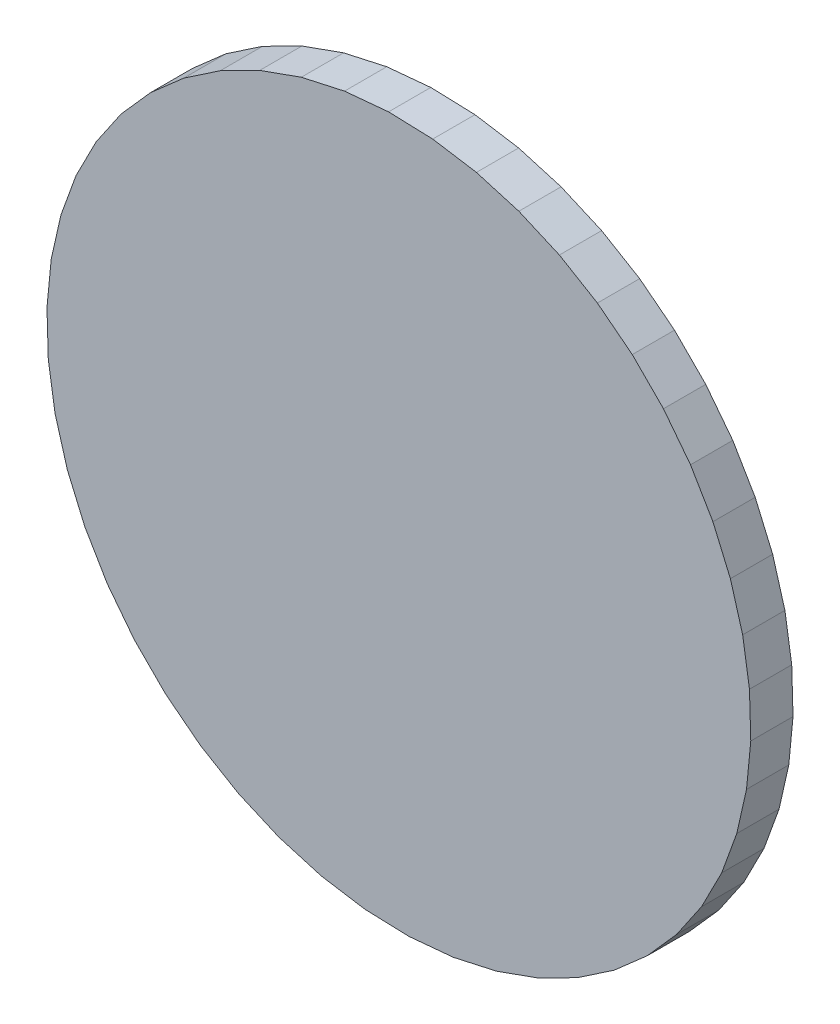
SolidWorks part; units mm, degrees
ref_plane "Front Plane" through (0, 0, 0) normal (0, 0, 1) x (1, 0, 0)
ref_plane "Top Plane" through (0, 0, 0) normal (0, 1, 0) x (1, 0, 0)
ref_plane "Right Plane" through (0, 0, 0) normal (1, 0, 0) x (0, 0, -1)
ref_plane "Plane1" through (0, 0, 36.0806) normal (0, 0, -1) x (-1, 0, 0)
sketch "Sketch1" plane through (0, 0, 36.0806) normal (0, 0, -1) x (-1, 0, 0)
  line L0 (24.986, 0.8369) -> (24.6841, 3.9619)
  line L1 (24.6841, 3.9619) -> (23.9929, 7.0244)
  line L2 (23.9929, 7.0244) -> (22.9233, 9.9761)
  line L3 (22.9233, 9.9761) -> (21.4922, 12.7705)
  line L4 (21.4922, 12.7705) -> (19.7222, 15.3635)
  line L5 (19.7222, 15.3635) -> (17.6411, 17.7142)
  line L6 (17.6411, 17.7142) -> (15.2818, 19.7855)
  line L7 (15.2818, 19.7855) -> (12.6816, 21.5448)
  line L8 (12.6816, 21.5448) -> (9.8813, 22.9643)
  line L9 (9.8813, 22.9643) -> (6.9252, 24.0217)
  line L10 (6.9252, 24.0217) -> (3.8598, 24.7002)
  line L11 (3.8598, 24.7002) -> (0.7336, 24.9892)
  line L12 (0.7336, 24.9892) -> (-2.4041, 24.8841)
  line L13 (-2.4041, 24.8841) -> (-5.504, 24.3866)
  line L14 (-5.504, 24.3866) -> (-8.517, 23.5045)
  line L15 (-8.517, 23.5045) -> (-11.3958, 22.2517)
  line L16 (-11.3958, 22.2517) -> (-14.0948, 20.6479)
  line L17 (-14.0948, 20.6479) -> (-16.5715, 18.7186)
  line L18 (-16.5715, 18.7186) -> (-18.7869, 16.494)
  line L19 (-18.7869, 16.494) -> (-20.706, 14.0093)
  line L20 (-20.706, 14.0093) -> (-22.2986, 11.3037)
  line L21 (-22.2986, 11.3037) -> (-23.5395, 8.4198)
  line L22 (-23.5395, 8.4198) -> (-24.4091, 5.4032)
  line L23 (-24.4091, 5.4032) -> (-24.8939, 2.3013)
  line L24 (-24.8939, 2.3013) -> (-24.986, -0.8369)
  line L25 (-24.986, -0.8369) -> (-24.6841, -3.9619)
  line L26 (-24.6841, -3.9619) -> (-23.9929, -7.0244)
  line L27 (-23.9929, -7.0244) -> (-22.9233, -9.9761)
  line L28 (-22.9233, -9.9761) -> (-21.4922, -12.7705)
  line L29 (-21.4922, -12.7705) -> (-19.7222, -15.3635)
  line L30 (-19.7222, -15.3635) -> (-17.6411, -17.7142)
  line L31 (-17.6411, -17.7142) -> (-15.2818, -19.7855)
  line L32 (-15.2818, -19.7855) -> (-12.6816, -21.5448)
  line L33 (-12.6816, -21.5448) -> (-9.8813, -22.9643)
  line L34 (-9.8813, -22.9643) -> (-6.9252, -24.0217)
  line L35 (-6.9252, -24.0217) -> (-3.8598, -24.7002)
  line L36 (-3.8598, -24.7002) -> (-0.7336, -24.9892)
  line L37 (-0.7336, -24.9892) -> (2.4041, -24.8841)
  line L38 (2.4041, -24.8841) -> (5.504, -24.3866)
  line L39 (5.504, -24.3866) -> (8.517, -23.5045)
  line L40 (8.517, -23.5045) -> (11.3958, -22.2517)
  line L41 (11.3958, -22.2517) -> (14.0948, -20.6479)
  line L42 (14.0948, -20.6479) -> (16.5715, -18.7186)
  line L43 (16.5715, -18.7186) -> (18.7869, -16.494)
  line L44 (18.7869, -16.494) -> (20.706, -14.0093)
  line L45 (20.706, -14.0093) -> (22.2986, -11.3037)
  line L46 (22.2986, -11.3037) -> (23.5395, -8.4198)
  line L47 (23.5395, -8.4198) -> (24.4091, -5.4032)
  line L48 (24.4091, -5.4032) -> (24.8939, -2.3013)
  line L49 (24.8939, -2.3013) -> (24.986, 0.8369)
extrude "Boss-Extrude1" add sketch "Sketch1" against normal blind 3
